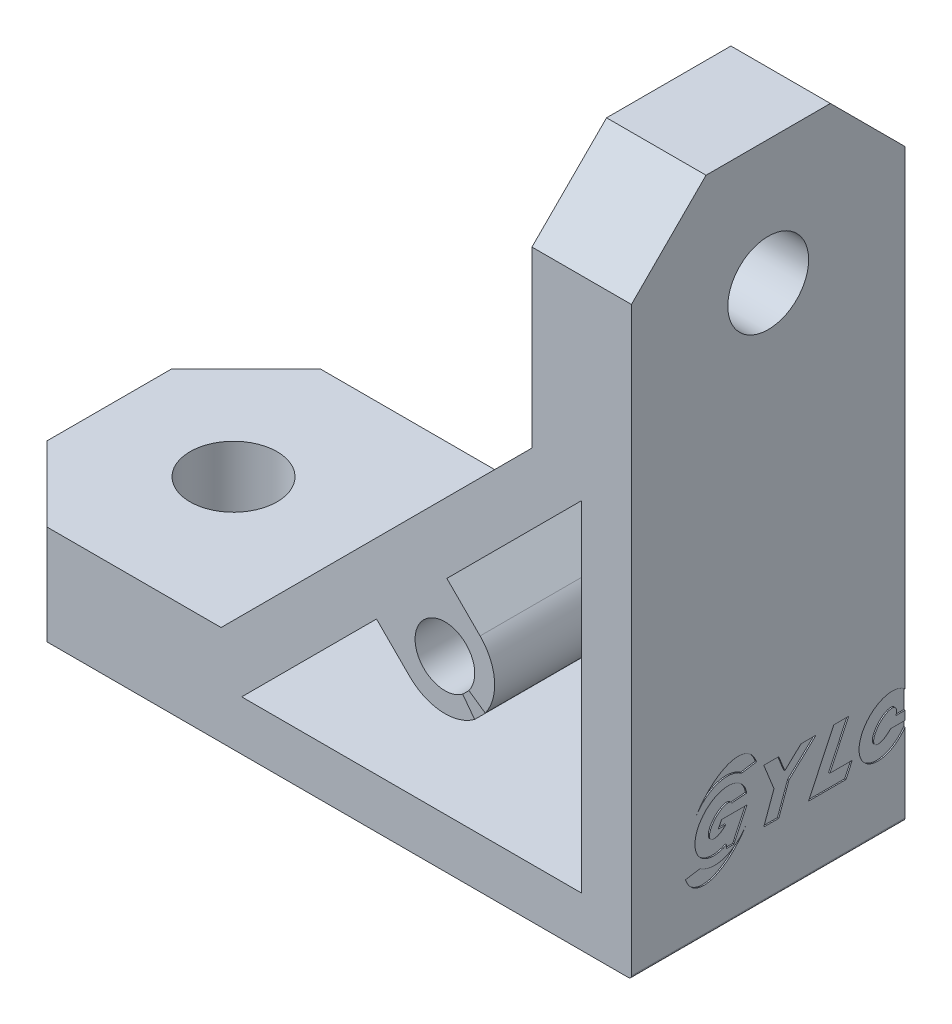
from build123d import *

# Parameters (mm, degrees)
EXTRUDE_1_DEPTH     = 22
SKETCH_1_R          = 3.5
CUT_EXTRUDE_1_DEPTH = 10
SKETCH_3_R          = 3.25
CUT_EXTRUDE_2_DEPTH = 10
CUT_EXTRUDE_3_DEPTH = 0.1
CHAMFER_2_SIZE      = 6


with BuildPart() as part:
    # Model → 凸台-拉伸1 (new body)
    with BuildSketch(Plane.XY):
        with BuildLine():
            Line((376.14070145, 195.588546008), (384.14070145, 195.588546008))
            Line((384.14070145, 195.588546008), (384.14070145, 142.825500368))
            ThreePointArc((384.14070145, 142.825500368), (384.071299125, 142.657948334), (383.90374709, 142.588546008))
            Line((383.90374709, 142.588546008), (331.14070145, 142.588546008))
            Line((331.14070145, 142.588546008), (331.14070145, 150.588546008))
            Line((331.14070145, 150.588546008), (351.14070145, 150.588546008))
            Line((351.14070145, 150.588546008), (376.14070145, 175.588546008))
            Line((376.14070145, 175.588546008), (376.14070145, 195.588546008))
        make_face()
        with BuildLine():
            Line((352.797555699, 146.588546008), (380.14070145, 146.588546008))
            Line((380.14070145, 146.588546008), (380.14070145, 173.931691759))
            Line((380.14070145, 173.931691759), (369.297555699, 163.088546008))
            Line((369.297555699, 163.088546008), (371.969128574, 160.416973133))
            ThreePointArc((371.969128574, 160.416973133), (373.12775021, 157.910170293), (372.385928963, 155.25006394))
            Line((372.385928963, 155.25006394), (371.072213777, 156.164024991))
            ThreePointArc((371.072213777, 156.164024991), (367.439726654, 159.281674694), (370.574137304, 155.663640387))
            Line((370.574137304, 155.663640387), (371.529761206, 154.380369972))
            ThreePointArc((371.529761206, 154.380369972), (368.850334045, 153.599099083), (366.312274325, 154.760118884))
            Line((366.312274325, 154.760118884), (363.64070145, 157.431691759))
            Line((363.64070145, 157.431691759), (352.797555699, 146.588546008))
        make_face(mode=Mode.SUBTRACT)
    extrude(amount=EXTRUDE_1_DEPTH)

    # 草图1 → 切除-拉伸1 (cut)
    with BuildSketch(Plane(origin=(0, 142.588546008, 0), x_dir=(-1, 0, 0), z_dir=(0, -1, 0))):
        with Locations(Location((-341.14070145, -11, 0), (0, 0, 90))):
            Circle(SKETCH_1_R)
        with Locations((-341.14070145, -41)):
            Circle(SKETCH_1_R)
    extrude(amount=-CUT_EXTRUDE_1_DEPTH, mode=Mode.SUBTRACT)

    # 草图3 → 切除-拉伸2 (cut)
    with BuildSketch(Plane(origin=(384.14070145, 0, 0), x_dir=(0, 0, -1), z_dir=(1, 0, 0))):
        with Locations((-11, 185.588546008)):
            Circle(SKETCH_3_R)
        with Locations((19, 185.588546008)):
            Circle(SKETCH_3_R)
    extrude(amount=-CUT_EXTRUDE_2_DEPTH, mode=Mode.SUBTRACT)

    # 草图4 → 切除-拉伸3 (cut)
    with BuildSketch(Plane(origin=(384.14070145, 0, 0), x_dir=(0, 0, -1), z_dir=(1, 0, 0))):
        with BuildLine():
            Line((-1.156910998, 149.620936237), (0.265081975, 149.620936237))
            add(Edge.make_bspline(
                [(0.472786894, 150.324263564), (0.930359486, 153.582209756), (-2.160166716, 151.852897671), (-5.250692919, 150.123585587), (-3.22217607, 148.256737296), (-1.193659222, 146.389889004), (0.265081975, 149.620936237)],
                knots=[2.310776883, 2.310776883, 2.310776883, 4.295504112, 4.295504112, 6.280231341, 6.280231341, 8.26495857, 8.26495857, 8.26495857], degree=2, weights=[1, 0.546712287, 1, 0.546712287, 1, 0.546712287, 1]))
            Line((0.472786894, 150.324263564), (-0.727213106, 150.324263564))
            add(Edge.make_bspline(
                [(-0.727213106, 150.324263564), (-0.331693937, 151.551759326), (-1.551251149, 150.835698352), (-2.770808361, 150.119637377), (-2.499443953, 149.28370119), (-2.228079545, 148.447765002), (-1.156910998, 149.620936237)],
                knots=[2.310776883, 2.310776883, 2.310776883, 4.1585118, 4.1585118, 6.006246717, 6.006246717, 7.853981634, 7.853981634, 7.853981634], degree=2, weights=[1, 0.602738677, 1, 0.602738677, 1, 0.602738677, 1]))
        make_face()
        with BuildLine():
            Line((-13.925569034, 150.826737427), (-12.730135397, 150.931324318))
            add(Edge.make_bspline(
                [(-12.730135397, 150.931324318), (-13.532943041, 155.84269164), (-16.525470552, 150.700825597), (-19.517998063, 145.558959554), (-14.356910998, 148.136141251)],
                knots=[2.606547406, 2.606547406, 2.606547406, 4.993026489, 4.993026489, 7.379505572, 7.379505572, 7.379505572], degree=2, weights=[1, 0.368650437, 1, 0.368650437, 1]))
            Line((-14.356910998, 148.136141251), (-14.356910998, 147.877409345))
            Line((-14.356910998, 147.877409345), (-13.756910998, 147.877409345))
            Line((-13.756910998, 147.877409345), (-12.713374, 150.089660335))
            Line((-12.713374, 150.089660335), (-14.741418493, 150.089660335))
            Line((-14.741418493, 150.089660335), (-15.017517564, 149.556960323))
            Line((-15.017517564, 149.556960323), (-14.417517564, 149.556960323))
            add(Edge.make_bspline(
                [(-13.925569034, 150.826737427), (-14.690411989, 152.268585428), (-15.646229095, 149.801508889), (-16.602046201, 147.334432349), (-14.417517564, 149.556960323)],
                knots=[2.964843337, 2.964843337, 2.964843337, 5.372666732, 5.372666732, 7.780490127, 7.780490127, 7.780490127], degree=2, weights=[1, 0.358709137, 1, 0.358709137, 1]))
        make_face()
        Polygon((-11.356910998, 147.877409345), (-10.156910998, 147.877409345), (-9.336062654, 150.132671635), (-7.156910998, 152.173591391), (-8.356910998, 152.173591391), (-9.664401992, 150.949039538), (-10.156910998, 152.173591391), (-11.356910998, 152.173591391), (-10.536062654, 150.132671635), align=None)
        Polygon((-5.73036657, 152.173591391), (-7.756910998, 147.877409345), (-4.756910998, 147.877409345), (-4.244959606, 148.96272302), (-6.044959606, 148.96272302), (-4.53036657, 152.173591391), align=None)
        with BuildLine():
            Line((-13.130690832, 152.515854721), (-11.945152764, 152.701595103))
            add(Edge.make_bspline(
                [(-11.945152764, 152.701595103), (-13.36499983, 157.051657906), (-16.85513293, 151.265027956)],
                knots=[2.682976295, 2.682976295, 2.682976295, 4.71238898, 4.71238898, 4.71238898], degree=2, weights=[1, 0.527869365, 1]))
            add(Edge.make_bspline(
                [(-13.130690832, 152.515854721), (-15.210313594, 153.992133359), (-16.85513293, 151.265027956)],
                knots=[3.081871514, 3.081871514, 3.081871514, 4.71238898, 4.71238898, 4.71238898], degree=2, weights=[1, 0.685680084, 1]))
        make_face()
        with BuildLine():
            Line((-17.654847236, 147.349405634), (-16.469309168, 147.535146015))
            add(Edge.make_bspline(
                [(-16.469309168, 147.535146015), (-14.389686406, 146.058867378), (-12.74486707, 148.78597278)],
                knots=[6.223464168, 6.223464168, 6.223464168, 7.853981634, 7.853981634, 7.853981634], degree=2, weights=[1, 0.685680084, 1]))
            add(Edge.make_bspline(
                [(-17.654847236, 147.349405634), (-16.23500017, 142.999342831), (-12.74486707, 148.78597278)],
                knots=[5.824568949, 5.824568949, 5.824568949, 7.853981634, 7.853981634, 7.853981634], degree=2, weights=[1, 0.527869365, 1]))
        make_face()
    extrude(amount=-CUT_EXTRUDE_3_DEPTH, mode=Mode.SUBTRACT)

    # 倒角2
    chamfer_2_edges = [part.edges().sort_by_distance(p)[0] for p in [
        (331.14070145, 146.588546008, 22),
        (380.14070145, 195.588546008, 22),
        (380.14070145, 195.588546008, 0),
        (331.14070145, 146.588546008, 0),
    ]]
    chamfer(chamfer_2_edges, length=CHAMFER_2_SIZE)


solid = part.part
